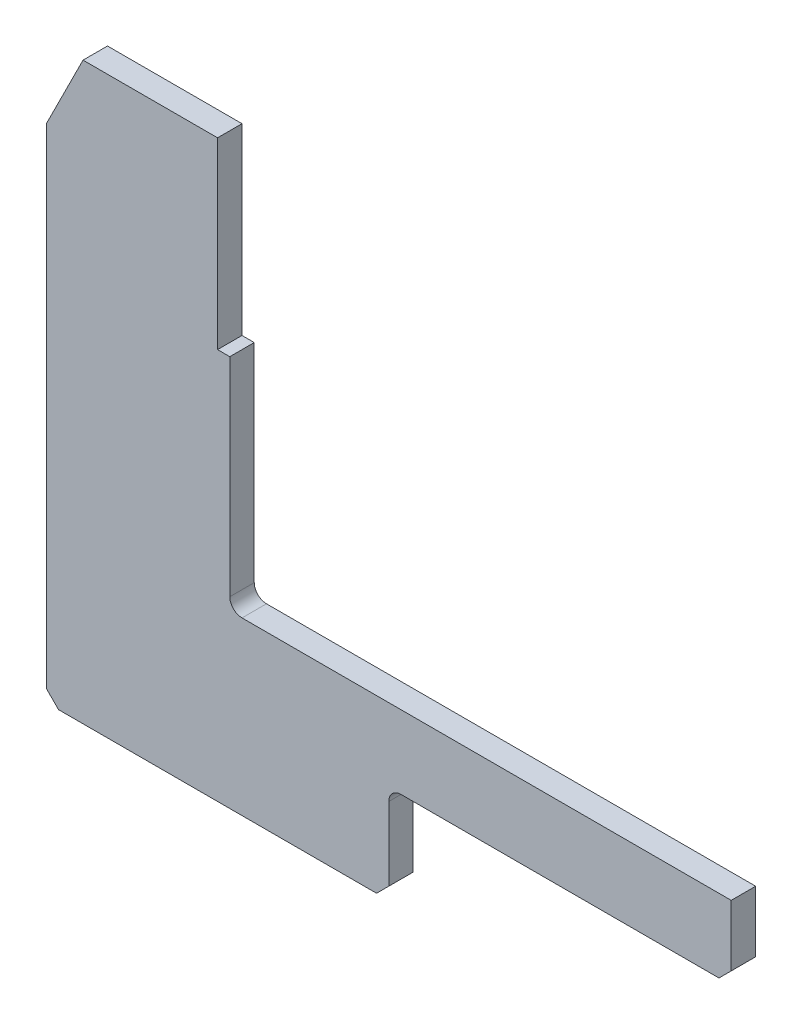
from build123d import *

# Parameters (mm, degrees)
BOSS_EXTRUDE1_DEPTH = 40
CHAMFER1_SIZE       = 20
FILLET1_R           = 20


with BuildPart() as part:
    # Sketch1 → Boss-Extrude1 (new body)
    with BuildSketch(Plane.XY):
        Polygon((-61.630811554, 752.729767781), (-61.630811554, -67.270232219), (498.369188446, -67.270232219), (498.369188446, 92.729767781), (1058.369188446, 92.729767781), (1058.369188446, 212.729767781), (238.369188446, 212.729767781), (238.369188446, 572.729767781), (218.369188446, 572.729767781), (218.369188446, 872.729767781), (-1.630811554, 872.729767781), align=None)
    extrude(amount=BOSS_EXTRUDE1_DEPTH)

    # Chamfer1
    chamfer1_edges = [part.edges().sort_by_distance(p)[0] for p in [
        (-61.630811554, -67.270232219, 20),
        (1058.369188446, 92.729767781, 20),
        (498.369188446, -67.270232219, 20),
    ]]
    chamfer(chamfer1_edges, length=CHAMFER1_SIZE)

    # Fillet1
    fillet1_edges = [part.edges().sort_by_distance(p)[0] for p in [
        (238.369188446, 212.729767781, 20),
        (498.369188446, 92.729767781, 20),
    ]]
    fillet(fillet1_edges, radius=FILLET1_R)


solid = part.part
